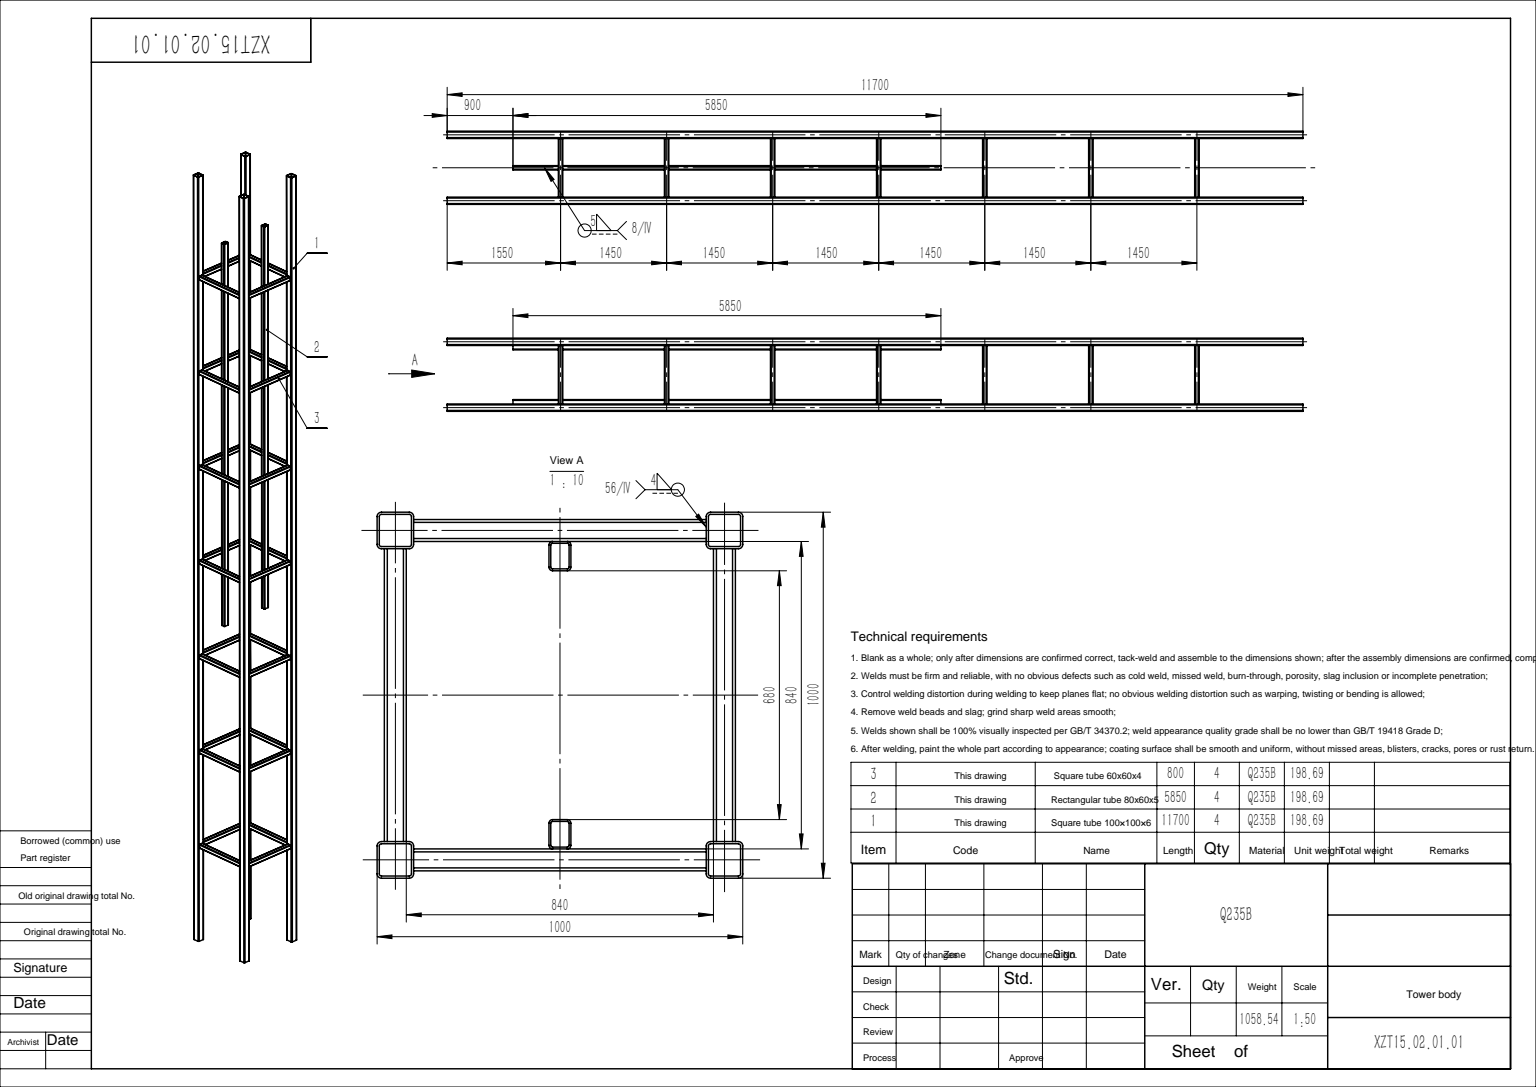
from build123d import *

# Parameters (mm, degrees)
GB_T_6728_2002_SQUARE_HOLLOW_SECTION_100_DEPTH = 11700
GB_T_6728_2002_SQUARE_HOLLOW_SECTION_2_DEPTH   = 11700
GB_T_6728_2002_SQUARE_HOLLOW_SECTION_3_DEPTH   = 11700
GB_T_6728_2002_SQUARE_HOLLOW_SECTION_4_DEPTH   = 11700
GB_T_6728_2002_SQUARE_HOLLOW_SECTION_60_DEPTH  = 900
GB_T_6728_2002_SQUARE_HOLLOW_SECTION_5_DEPTH   = 900
GB_T_6728_2002_SQUARE_HOLLOW_SECTION_6_DEPTH   = 900
GB_T_6728_2002_SQUARE_HOLLOW_SECTION_7_DEPTH   = 900
GB_T_6728_2002_RECTANGULAR_HOLLOW_SECTIO_DEPTH = 5850
GB_T_6728_2002_RECTANGULAR_HOLLOW_SE_2_DEPTH   = 5850
LINEARPATTERN1_COUNT                           = 7
LINEARPATTERN1_PITCH                           = 1450


with BuildPart() as part:
    # Sketch1 → GB/T 6728-2002 square hollow section 100×100×6(1) (new body)
    with BuildSketch(Plane(origin=(-450, 0, -450), x_dir=(1, 0, 0), z_dir=(0, 1, 0))):
        with BuildLine():
            Line((-38, -50), (38, -50))
            ThreePointArc((38, -50), (46.485281374, -46.485281374), (50, -38))
            Line((50, -38), (50, 38))
            ThreePointArc((50, 38), (46.485281374, 46.485281374), (38, 50))
            Line((38, 50), (-38, 50))
            ThreePointArc((-38, 50), (-46.485281374, 46.485281374), (-50, 38))
            Line((-50, 38), (-50, -38))
            ThreePointArc((-50, -38), (-46.485281374, -46.485281374), (-38, -50))
        make_face()
        with BuildLine():
            Line((-38, -44), (38, -44))
            ThreePointArc((38, -44), (42.242640687, -42.242640687), (44, -38))
            Line((44, -38), (44, 38))
            ThreePointArc((44, 38), (42.242640687, 42.242640687), (38, 44))
            Line((38, 44), (-38, 44))
            ThreePointArc((-38, 44), (-42.242640687, 42.242640687), (-44, 38))
            Line((-44, 38), (-44, -38))
            ThreePointArc((-44, -38), (-42.242640687, -42.242640687), (-38, -44))
        make_face(mode=Mode.SUBTRACT)
    extrude(amount=GB_T_6728_2002_SQUARE_HOLLOW_SECTION_100_DEPTH)


with BuildPart() as body_2:
    # Sketch1 on segment 2 (carried to segment 2) → GB_T 6728-2002 square hollow section 2 (new body)
    with BuildSketch(Plane(origin=(-450, 0, 450), x_dir=(1, 0, 0), z_dir=(0, 1, 0))):
        with BuildLine():
            Line((-38, -50), (38, -50))
            ThreePointArc((38, -50), (46.485281374, -46.485281374), (50, -38))
            Line((50, -38), (50, 38))
            ThreePointArc((50, 38), (46.485281374, 46.485281374), (38, 50))
            Line((38, 50), (-38, 50))
            ThreePointArc((-38, 50), (-46.485281374, 46.485281374), (-50, 38))
            Line((-50, 38), (-50, -38))
            ThreePointArc((-50, -38), (-46.485281374, -46.485281374), (-38, -50))
        make_face()
        with BuildLine():
            Line((-38, -44), (38, -44))
            ThreePointArc((38, -44), (42.242640687, -42.242640687), (44, -38))
            Line((44, -38), (44, 38))
            ThreePointArc((44, 38), (42.242640687, 42.242640687), (38, 44))
            Line((38, 44), (-38, 44))
            ThreePointArc((-38, 44), (-42.242640687, 42.242640687), (-44, 38))
            Line((-44, 38), (-44, -38))
            ThreePointArc((-44, -38), (-42.242640687, -42.242640687), (-38, -44))
        make_face(mode=Mode.SUBTRACT)
    extrude(amount=GB_T_6728_2002_SQUARE_HOLLOW_SECTION_2_DEPTH)


with BuildPart() as body_3:
    # Sketch1 on segment 3 (carried to segment 3) → GB_T 6728-2002 square hollow section 3 (new body)
    with BuildSketch(Plane(origin=(450, 0, 450), x_dir=(1, 0, 0), z_dir=(0, 1, 0))):
        with BuildLine():
            Line((-38, -50), (38, -50))
            ThreePointArc((38, -50), (46.485281374, -46.485281374), (50, -38))
            Line((50, -38), (50, 38))
            ThreePointArc((50, 38), (46.485281374, 46.485281374), (38, 50))
            Line((38, 50), (-38, 50))
            ThreePointArc((-38, 50), (-46.485281374, 46.485281374), (-50, 38))
            Line((-50, 38), (-50, -38))
            ThreePointArc((-50, -38), (-46.485281374, -46.485281374), (-38, -50))
        make_face()
        with BuildLine():
            Line((-38, -44), (38, -44))
            ThreePointArc((38, -44), (42.242640687, -42.242640687), (44, -38))
            Line((44, -38), (44, 38))
            ThreePointArc((44, 38), (42.242640687, 42.242640687), (38, 44))
            Line((38, 44), (-38, 44))
            ThreePointArc((-38, 44), (-42.242640687, 42.242640687), (-44, 38))
            Line((-44, 38), (-44, -38))
            ThreePointArc((-44, -38), (-42.242640687, -42.242640687), (-38, -44))
        make_face(mode=Mode.SUBTRACT)
    extrude(amount=GB_T_6728_2002_SQUARE_HOLLOW_SECTION_3_DEPTH)


with BuildPart() as body_4:
    # Sketch1 on segment 4 (carried to segment 4) → GB_T 6728-2002 square hollow section 4 (new body)
    with BuildSketch(Plane(origin=(450, 0, -450), x_dir=(1, 0, 0), z_dir=(0, 1, 0))):
        with BuildLine():
            Line((-38, -50), (38, -50))
            ThreePointArc((38, -50), (46.485281374, -46.485281374), (50, -38))
            Line((50, -38), (50, 38))
            ThreePointArc((50, 38), (46.485281374, 46.485281374), (38, 50))
            Line((38, 50), (-38, 50))
            ThreePointArc((-38, 50), (-46.485281374, 46.485281374), (-50, 38))
            Line((-50, 38), (-50, -38))
            ThreePointArc((-50, -38), (-46.485281374, -46.485281374), (-38, -50))
        make_face()
        with BuildLine():
            Line((-38, -44), (38, -44))
            ThreePointArc((38, -44), (42.242640687, -42.242640687), (44, -38))
            Line((44, -38), (44, 38))
            ThreePointArc((44, 38), (42.242640687, 42.242640687), (38, 44))
            Line((38, 44), (-38, 44))
            ThreePointArc((-38, 44), (-42.242640687, 42.242640687), (-44, 38))
            Line((-44, 38), (-44, -38))
            ThreePointArc((-44, -38), (-42.242640687, -42.242640687), (-38, -44))
        make_face(mode=Mode.SUBTRACT)
    extrude(amount=GB_T_6728_2002_SQUARE_HOLLOW_SECTION_4_DEPTH)


with BuildPart() as body_5:
    # Sketch12 → GB/T 6728-2002 square hollow section 60×60×4(1) (new body)
    with BuildSketch(Plane(origin=(-450, 1550, -450), x_dir=(1, 0, 0), z_dir=(0, 0, 1))):
        with BuildLine():
            Line((-22, -30), (22, -30))
            ThreePointArc((22, -30), (27.656854249, -27.656854249), (30, -22))
            Line((30, -22), (30, 22))
            ThreePointArc((30, 22), (27.656854249, 27.656854249), (22, 30))
            Line((22, 30), (-22, 30))
            ThreePointArc((-22, 30), (-27.656854249, 27.656854249), (-30, 22))
            Line((-30, 22), (-30, -22))
            ThreePointArc((-30, -22), (-27.656854249, -27.656854249), (-22, -30))
        make_face()
        with BuildLine():
            Line((-22, -26), (22, -26))
            ThreePointArc((22, -26), (24.828427125, -24.828427125), (26, -22))
            Line((26, -22), (26, 22))
            ThreePointArc((26, 22), (24.828427125, 24.828427125), (22, 26))
            Line((22, 26), (-22, 26))
            ThreePointArc((-22, 26), (-24.828427125, 24.828427125), (-26, 22))
            Line((-26, 22), (-26, -22))
            ThreePointArc((-26, -22), (-24.828427125, -24.828427125), (-22, -26))
        make_face(mode=Mode.SUBTRACT)
    extrude(amount=GB_T_6728_2002_SQUARE_HOLLOW_SECTION_60_DEPTH)

    # Trim_Extend1 5
    split(bisect_by=Plane(origin=(-450, 5850, -400), x_dir=(0, -1, 0), z_dir=(0, 0, 1)), keep=Keep.TOP)

    # Trim_Extend1 50
    split(bisect_by=Plane(origin=(-450, 5850, 400), x_dir=(0, 1, 0), z_dir=(0, 0, -1)), keep=Keep.TOP)


with BuildPart() as body_6:
    # Sketch12 on segment 2 (carried to segment 2) → GB_T 6728-2002 square hollow section 5 (new body)
    with BuildSketch(Plane(origin=(-450, 1550, 450), x_dir=(0, 0, -1), z_dir=(1, 0, 0))):
        with BuildLine():
            Line((-22, -30), (22, -30))
            ThreePointArc((22, -30), (27.656854249, -27.656854249), (30, -22))
            Line((30, -22), (30, 22))
            ThreePointArc((30, 22), (27.656854249, 27.656854249), (22, 30))
            Line((22, 30), (-22, 30))
            ThreePointArc((-22, 30), (-27.656854249, 27.656854249), (-30, 22))
            Line((-30, 22), (-30, -22))
            ThreePointArc((-30, -22), (-27.656854249, -27.656854249), (-22, -30))
        make_face()
        with BuildLine():
            Line((-22, -26), (22, -26))
            ThreePointArc((22, -26), (24.828427125, -24.828427125), (26, -22))
            Line((26, -22), (26, 22))
            ThreePointArc((26, 22), (24.828427125, 24.828427125), (22, 26))
            Line((22, 26), (-22, 26))
            ThreePointArc((-22, 26), (-24.828427125, 24.828427125), (-26, 22))
            Line((-26, 22), (-26, -22))
            ThreePointArc((-26, -22), (-24.828427125, -24.828427125), (-22, -26))
        make_face(mode=Mode.SUBTRACT)
    extrude(amount=GB_T_6728_2002_SQUARE_HOLLOW_SECTION_5_DEPTH)

    # Trim/Extend1
    split(bisect_by=Plane(origin=(-400, 5850, -450), x_dir=(0, 1, 0), z_dir=(1, 0, 0)), keep=Keep.TOP)

    # Trim_Extend1 97
    split(bisect_by=Plane(origin=(400, 5850, 450), x_dir=(0, -1, 0), z_dir=(-1, 0, 0)), keep=Keep.TOP)


with BuildPart() as body_7:
    # Sketch12 on segment 3 (carried to segment 3) → GB_T 6728-2002 square hollow section 6 (new body)
    with BuildSketch(Plane(origin=(450, 1550, 450), x_dir=(-1, 0, 0), z_dir=(0, 0, -1))):
        with BuildLine():
            Line((-22, -30), (22, -30))
            ThreePointArc((22, -30), (27.656854249, -27.656854249), (30, -22))
            Line((30, -22), (30, 22))
            ThreePointArc((30, 22), (27.656854249, 27.656854249), (22, 30))
            Line((22, 30), (-22, 30))
            ThreePointArc((-22, 30), (-27.656854249, 27.656854249), (-30, 22))
            Line((-30, 22), (-30, -22))
            ThreePointArc((-30, -22), (-27.656854249, -27.656854249), (-22, -30))
        make_face()
        with BuildLine():
            Line((-22, -26), (22, -26))
            ThreePointArc((22, -26), (24.828427125, -24.828427125), (26, -22))
            Line((26, -22), (26, 22))
            ThreePointArc((26, 22), (24.828427125, 24.828427125), (22, 26))
            Line((22, 26), (-22, 26))
            ThreePointArc((-22, 26), (-24.828427125, 24.828427125), (-26, 22))
            Line((-26, 22), (-26, -22))
            ThreePointArc((-26, -22), (-24.828427125, -24.828427125), (-22, -26))
        make_face(mode=Mode.SUBTRACT)
    extrude(amount=GB_T_6728_2002_SQUARE_HOLLOW_SECTION_6_DEPTH)

    # Trim_Extend1 5
    split(bisect_by=Plane(origin=(-450, 5850, -400), x_dir=(0, -1, 0), z_dir=(0, 0, 1)), keep=Keep.TOP)

    # Trim_Extend1 86
    split(bisect_by=Plane.YX.offset(-400), keep=Keep.TOP)


with BuildPart() as body_8:
    # Sketch12 on segment 4 (carried to segment 4) → GB_T 6728-2002 square hollow section 7 (new body)
    with BuildSketch(Plane(origin=(450, 1550, -450), x_dir=(0, 0, 1), z_dir=(-1, 0, 0))):
        with BuildLine():
            Line((-22, -30), (22, -30))
            ThreePointArc((22, -30), (27.656854249, -27.656854249), (30, -22))
            Line((30, -22), (30, 22))
            ThreePointArc((30, 22), (27.656854249, 27.656854249), (22, 30))
            Line((22, 30), (-22, 30))
            ThreePointArc((-22, 30), (-27.656854249, 27.656854249), (-30, 22))
            Line((-30, 22), (-30, -22))
            ThreePointArc((-30, -22), (-27.656854249, -27.656854249), (-22, -30))
        make_face()
        with BuildLine():
            Line((-22, -26), (22, -26))
            ThreePointArc((22, -26), (24.828427125, -24.828427125), (26, -22))
            Line((26, -22), (26, 22))
            ThreePointArc((26, 22), (24.828427125, 24.828427125), (22, 26))
            Line((22, 26), (-22, 26))
            ThreePointArc((-22, 26), (-24.828427125, 24.828427125), (-26, 22))
            Line((-26, 22), (-26, -22))
            ThreePointArc((-26, -22), (-24.828427125, -24.828427125), (-22, -26))
        make_face(mode=Mode.SUBTRACT)
    extrude(amount=GB_T_6728_2002_SQUARE_HOLLOW_SECTION_7_DEPTH)

    # Trim/Extend1
    split(bisect_by=Plane(origin=(-400, 5850, -450), x_dir=(0, 1, 0), z_dir=(1, 0, 0)), keep=Keep.TOP)

    # Trim_Extend1 97
    split(bisect_by=Plane(origin=(400, 5850, 450), x_dir=(0, -1, 0), z_dir=(-1, 0, 0)), keep=Keep.TOP)


with BuildPart() as body_9:
    # Sketch14 → GB/T 6728-2002 rectangular hollow section 80X60X5(1) (new body)
    with BuildSketch(Plane(origin=(-380, 900, 0), x_dir=(0, 0, -1), z_dir=(0, 1, 0))):
        with BuildLine():
            Line((-20, -40), (20, -40))
            ThreePointArc((20, -40), (27.071067812, -37.071067812), (30, -30))
            Line((30, -30), (30, 30))
            ThreePointArc((30, 30), (27.071067812, 37.071067812), (20, 40))
            Line((20, 40), (-20, 40))
            ThreePointArc((-20, 40), (-27.071067812, 37.071067812), (-30, 30))
            Line((-30, 30), (-30, -30))
            ThreePointArc((-30, -30), (-27.071067812, -37.071067812), (-20, -40))
        make_face()
        with BuildLine():
            Line((-20, -35), (20, -35))
            ThreePointArc((20, -35), (23.535533906, -33.535533906), (25, -30))
            Line((25, -30), (25, 30))
            ThreePointArc((25, 30), (23.535533906, 33.535533906), (20, 35))
            Line((20, 35), (-20, 35))
            ThreePointArc((-20, 35), (-23.535533906, 33.535533906), (-25, 30))
            Line((-25, 30), (-25, -30))
            ThreePointArc((-25, -30), (-23.535533906, -33.535533906), (-20, -35))
        make_face(mode=Mode.SUBTRACT)
    extrude(amount=GB_T_6728_2002_RECTANGULAR_HOLLOW_SECTIO_DEPTH)


with BuildPart() as body_10:
    # Sketch14 on segment 2 (carried to segment 2) → GB_T 6728-2002 rectangular hollow se 2 (new body)
    with BuildSketch(Plane(origin=(380, 900, 0), x_dir=(0, 0, -1), z_dir=(0, 1, 0))):
        with BuildLine():
            Line((-20, -40), (20, -40))
            ThreePointArc((20, -40), (27.071067812, -37.071067812), (30, -30))
            Line((30, -30), (30, 30))
            ThreePointArc((30, 30), (27.071067812, 37.071067812), (20, 40))
            Line((20, 40), (-20, 40))
            ThreePointArc((-20, 40), (-27.071067812, 37.071067812), (-30, 30))
            Line((-30, 30), (-30, -30))
            ThreePointArc((-30, -30), (-27.071067812, -37.071067812), (-20, -40))
        make_face()
        with BuildLine():
            Line((-20, -35), (20, -35))
            ThreePointArc((20, -35), (23.535533906, -33.535533906), (25, -30))
            Line((25, -30), (25, 30))
            ThreePointArc((25, 30), (23.535533906, 33.535533906), (20, 35))
            Line((20, 35), (-20, 35))
            ThreePointArc((-20, 35), (-23.535533906, 33.535533906), (-25, 30))
            Line((-25, 30), (-25, -30))
            ThreePointArc((-25, -30), (-23.535533906, -33.535533906), (-20, -35))
        make_face(mode=Mode.SUBTRACT)
    extrude(amount=GB_T_6728_2002_RECTANGULAR_HOLLOW_SE_2_DEPTH)


with BuildPart() as linearpattern1_1:
    # LinearPattern1: pattern copy
    add(body_7.part.moved(Location(Vector(0, 1, 0) * (1 * LINEARPATTERN1_PITCH))))


with BuildPart() as linearpattern1_2:
    # LinearPattern1: pattern copy
    add(body_7.part.moved(Location(Vector(0, 1, 0) * (2 * LINEARPATTERN1_PITCH))))


with BuildPart() as linearpattern1_3:
    # LinearPattern1: pattern copy
    add(body_7.part.moved(Location(Vector(0, 1, 0) * (3 * LINEARPATTERN1_PITCH))))


with BuildPart() as linearpattern1_4:
    # LinearPattern1: pattern copy
    add(body_7.part.moved(Location(Vector(0, 1, 0) * (4 * LINEARPATTERN1_PITCH))))


with BuildPart() as linearpattern1_5:
    # LinearPattern1: pattern copy
    add(body_7.part.moved(Location(Vector(0, 1, 0) * (5 * LINEARPATTERN1_PITCH))))


with BuildPart() as linearpattern1_6:
    # LinearPattern1: pattern copy
    add(body_7.part.moved(Location(Vector(0, 1, 0) * (6 * LINEARPATTERN1_PITCH))))


with BuildPart() as linearpattern1_7:
    # LinearPattern1: pattern copy
    add(body_6.part.moved(Location(Vector(0, 1, 0) * (1 * LINEARPATTERN1_PITCH))))


with BuildPart() as linearpattern1_8:
    # LinearPattern1: pattern copy
    add(body_6.part.moved(Location(Vector(0, 1, 0) * (2 * LINEARPATTERN1_PITCH))))


with BuildPart() as linearpattern1_9:
    # LinearPattern1: pattern copy
    add(body_6.part.moved(Location(Vector(0, 1, 0) * (3 * LINEARPATTERN1_PITCH))))


with BuildPart() as linearpattern1_10:
    # LinearPattern1: pattern copy
    add(body_6.part.moved(Location(Vector(0, 1, 0) * (4 * LINEARPATTERN1_PITCH))))


with BuildPart() as linearpattern1_11:
    # LinearPattern1: pattern copy
    add(body_6.part.moved(Location(Vector(0, 1, 0) * (5 * LINEARPATTERN1_PITCH))))


with BuildPart() as linearpattern1_12:
    # LinearPattern1: pattern copy
    add(body_6.part.moved(Location(Vector(0, 1, 0) * (6 * LINEARPATTERN1_PITCH))))


with BuildPart() as linearpattern1_13:
    # LinearPattern1: pattern copy
    add(body_8.part.moved(Location(Vector(0, 1, 0) * (1 * LINEARPATTERN1_PITCH))))


with BuildPart() as linearpattern1_14:
    # LinearPattern1: pattern copy
    add(body_8.part.moved(Location(Vector(0, 1, 0) * (2 * LINEARPATTERN1_PITCH))))


with BuildPart() as linearpattern1_15:
    # LinearPattern1: pattern copy
    add(body_8.part.moved(Location(Vector(0, 1, 0) * (3 * LINEARPATTERN1_PITCH))))


with BuildPart() as linearpattern1_16:
    # LinearPattern1: pattern copy
    add(body_8.part.moved(Location(Vector(0, 1, 0) * (4 * LINEARPATTERN1_PITCH))))


with BuildPart() as linearpattern1_17:
    # LinearPattern1: pattern copy
    add(body_8.part.moved(Location(Vector(0, 1, 0) * (5 * LINEARPATTERN1_PITCH))))


with BuildPart() as linearpattern1_18:
    # LinearPattern1: pattern copy
    add(body_8.part.moved(Location(Vector(0, 1, 0) * (6 * LINEARPATTERN1_PITCH))))


with BuildPart() as linearpattern1_19:
    # LinearPattern1: pattern copy
    add(body_5.part.moved(Location(Vector(0, 1, 0) * (1 * LINEARPATTERN1_PITCH))))


with BuildPart() as linearpattern1_20:
    # LinearPattern1: pattern copy
    add(body_5.part.moved(Location(Vector(0, 1, 0) * (2 * LINEARPATTERN1_PITCH))))


with BuildPart() as linearpattern1_21:
    # LinearPattern1: pattern copy
    add(body_5.part.moved(Location(Vector(0, 1, 0) * (3 * LINEARPATTERN1_PITCH))))


with BuildPart() as linearpattern1_22:
    # LinearPattern1: pattern copy
    add(body_5.part.moved(Location(Vector(0, 1, 0) * (4 * LINEARPATTERN1_PITCH))))


with BuildPart() as linearpattern1_23:
    # LinearPattern1: pattern copy
    add(body_5.part.moved(Location(Vector(0, 1, 0) * (5 * LINEARPATTERN1_PITCH))))


with BuildPart() as linearpattern1_24:
    # LinearPattern1: pattern copy
    add(body_5.part.moved(Location(Vector(0, 1, 0) * (6 * LINEARPATTERN1_PITCH))))


solid = Compound([part.part, body_2.part, body_3.part, body_4.part, body_5.part, body_6.part, body_7.part, body_8.part, body_9.part, body_10.part, linearpattern1_1.part, linearpattern1_2.part, linearpattern1_3.part, linearpattern1_4.part, linearpattern1_5.part, linearpattern1_6.part, linearpattern1_7.part, linearpattern1_8.part, linearpattern1_9.part, linearpattern1_10.part, linearpattern1_11.part, linearpattern1_12.part, linearpattern1_13.part, linearpattern1_14.part, linearpattern1_15.part, linearpattern1_16.part, linearpattern1_17.part, linearpattern1_18.part, linearpattern1_19.part, linearpattern1_20.part, linearpattern1_21.part, linearpattern1_22.part, linearpattern1_23.part, linearpattern1_24.part])
